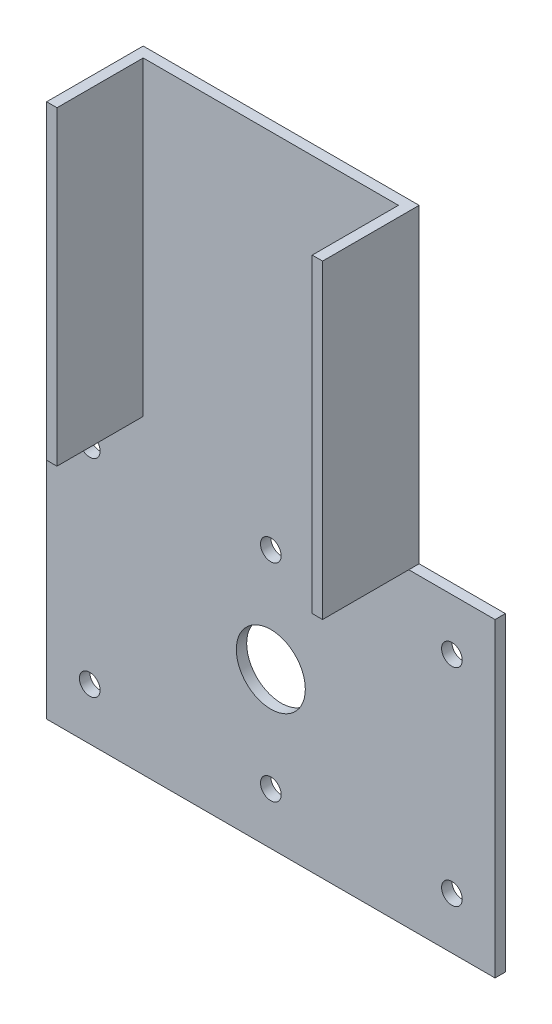
from build123d import *

# Parameters (mm, degrees)
SKETCH_1_W          = 80
SKETCH_1_H          = 90
SKETCH_1_W_2        = 130
EXTRUDE_1_DEPTH     = 3
SKETCH_2_W          = 3
SKETCH_2_H          = 90
EXTRUDE_2_DEPTH     = 25
SKETCH_3_R          = 10
SKETCH_3_R_2        = 3
CUT_EXTRUDE_1_DEPTH = 25


with BuildPart() as part:
    # 草图1 → 凸台-拉伸1 (new body)
    with BuildSketch(Plane.XY):
        with Locations((-65, 135)):
            Rectangle(SKETCH_1_W, SKETCH_1_H)
        with Locations((-65, 45)):
            Rectangle(SKETCH_1_W_2, SKETCH_1_H)
    extrude(amount=EXTRUDE_1_DEPTH)

    # 草图2 → 凸台-拉伸2 (add)
    with BuildSketch(Plane.XY.offset(3)):
        with Locations((-103.5, 135)):
            Rectangle(SKETCH_2_W, SKETCH_2_H)
        with Locations((-26.5, 135)):
            Rectangle(SKETCH_2_W, SKETCH_2_H)
    extrude(amount=EXTRUDE_2_DEPTH)

    # 草图3 → 切除-拉伸1 (cut)
    with BuildSketch(Plane(origin=(0, 0, 0), x_dir=(-1, 0, 0), z_dir=(0, 0, -1))):
        with Locations((65, 45)):
            Circle(SKETCH_3_R)
        with Locations((12.5, 15)):
            Circle(SKETCH_3_R_2)
        with Locations((65, 15)):
            Circle(SKETCH_3_R_2)
        with Locations((117.5, 15)):
            Circle(SKETCH_3_R_2)
        with Locations((117.5, 75)):
            Circle(SKETCH_3_R_2)
        with Locations((65, 75)):
            Circle(SKETCH_3_R_2)
        with Locations((12.5, 75)):
            Circle(SKETCH_3_R_2)
    extrude(amount=-CUT_EXTRUDE_1_DEPTH, mode=Mode.SUBTRACT)


solid = part.part
